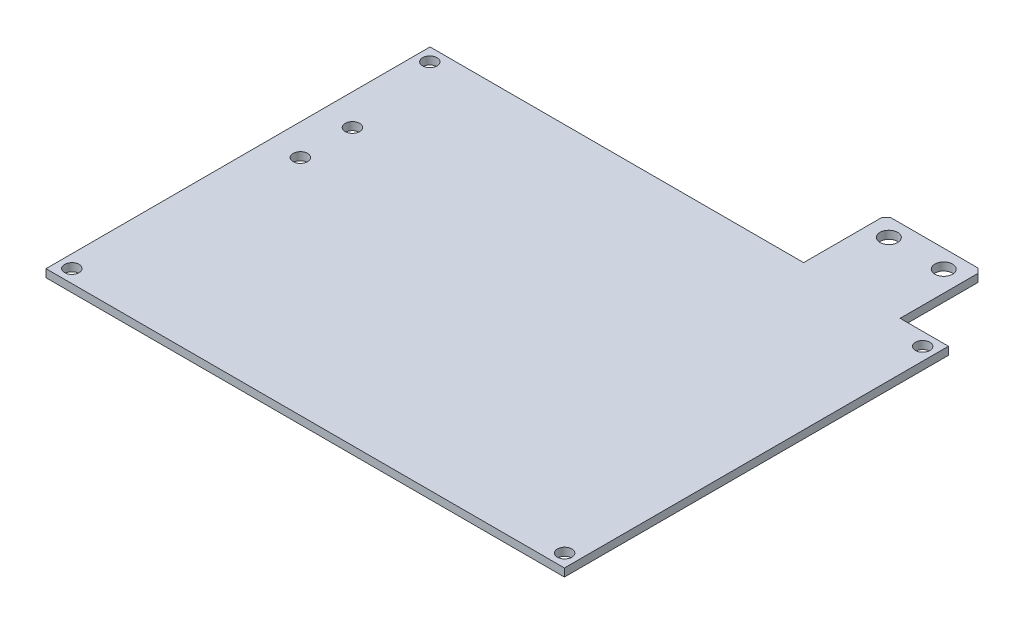
SolidWorks part; units mm, degrees
ref_plane "前视基准面" through (0, 0, 0) normal (0, 0, 1) x (1, 0, 0)
ref_plane "上视基准面" through (0, 0, 0) normal (0, 1, 0) x (1, 0, 0)
ref_plane "右视基准面" through (0, 0, 0) normal (1, 0, 0) x (0, 0, -1)
sketch "草图1" plane through (0, 0, 0) normal (0, 1, 0) x (1, 0, 0)
  line L0 (-55.75, 0) -> (55.75, 0) construction
  line L1 (-55.75, -41.3) -> (55.75, -41.3)
  line L2 (-55.75, -41.3) -> (-55.75, 41.3)
  line L3 (-55.75, 41.3) -> (24.6, 41.3)
  line L4 (55.75, -41.3) -> (55.75, 41.3)
  line L5 (-55.75, -41.3) -> (55.75, 41.3) construction
  line L6 (-55.75, 41.3) -> (55.75, -41.3) construction
  line L7 (0, 41.3) -> (0, -41.3) construction
  line L8 (24.6, 41.3) -> (24.6, 58.05)
  line L9 (25.6, 59.05) -> (44.35, 59.05)
  line L10 (45.35, 58.05) -> (45.35, 41.3)
  line L11 (45.35, 41.3) -> (55.75, 41.3)
  line L12 (34.975, 59.05) -> (34.975, 41.3) construction
  line L13 (24.6, 58.05) -> (25.6, 59.05)
  line L14 (44.35, 59.05) -> (45.35, 58.05)
  circle A0 centre (-53, 38.5) radius 1.55
  circle A1 centre (53, 38.5) radius 1.55
  circle A2 centre (53, -38.5) radius 1.55
  circle A3 centre (-53, -38.5) radius 1.55
  circle A4 centre (29.075, 55.15) radius 1.9
  circle A5 centre (40.875, 55.15) radius 1.9
  circle A6 centre (-49.1, 17.95) radius 1.55
  circle A7 centre (-49.1, 6.75) radius 1.55
  point P0 (0, 0)
  point P19 (24.6, 59.05)
  point P21 (45.35, 59.05)
  dimension "D3" = 3.1
  dimension "D8" = 10.4
  dimension "D9" = 3.8
  dimension "D10" = 2
  dimension "D12" = 5.1
  dimension "D13" = 5.1
  dimension "D14" = 21.8
  dimension "D15" = 33
  dimension "D1" = 82.6
  dimension "D2" = 111.5
  dimension "D4" = 106
  dimension "D5" = 77
  dimension "D6" = 20.75
  dimension "D7" = 17.75
  dimension "D11" = 11.8
extrude "凸台-拉伸1" add sketch "草图1" along normal blind 1.7
